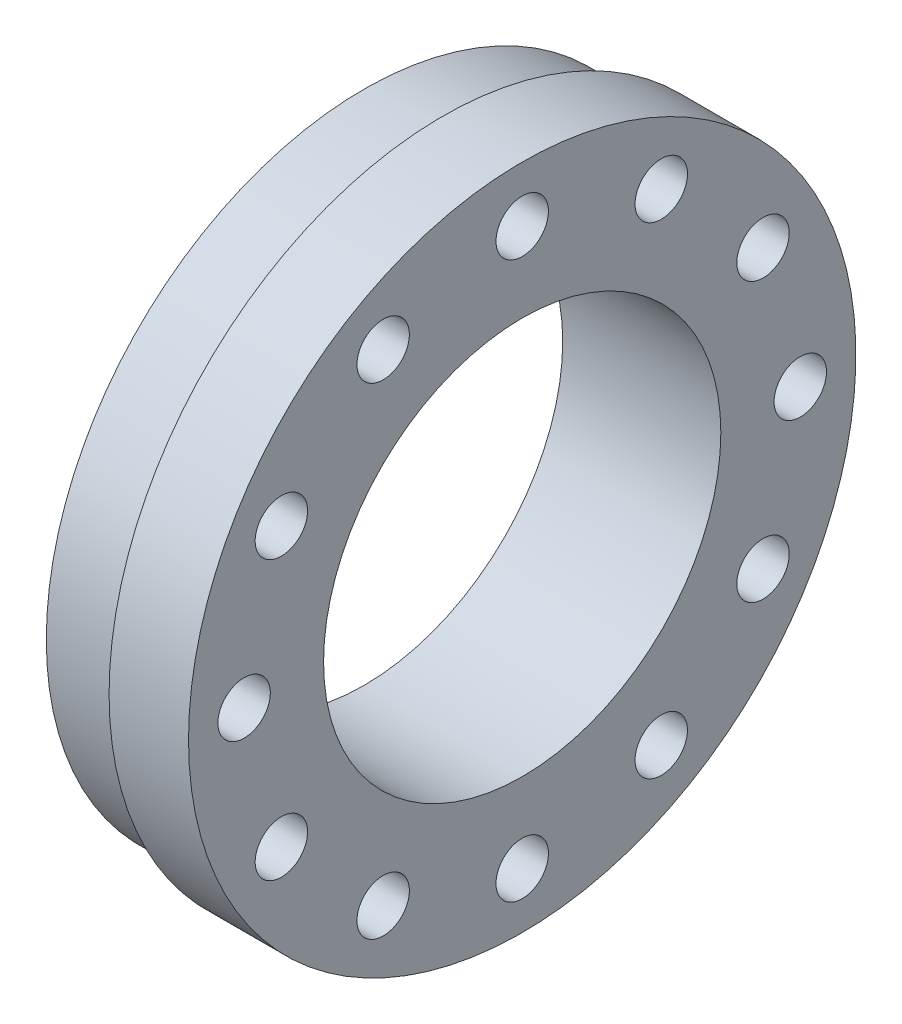
from build123d import *

# Parameters (mm, degrees)
HOLE_WIZARD_M4_1_D = 3.3


with BuildPart() as part:
    # 草图1 → 旋转1 (revolve)
    with BuildSketch(Plane(origin=(0, 0, 0), x_dir=(1, 0, 0), z_dir=(0, 1, 0)), mode=Mode.PRIVATE) as revolve_1_sk:
        Polygon((0, 12.5), (0, 20), (4.95, 20), (4.95, 21), (9.95, 21), (9.95, 12.5), align=None)
    revolve(revolve_1_sk.sketch.rotate(Axis((-63.943599205, 0, 0), (1, 0, 0)), 180), axis=Axis((-63.943599205, 0, 0), (1, 0, 0)))

    # M4 螺纹孔1 (through all)
    with Locations(Plane(origin=(9.95, 0, 0), x_dir=(0, 0, -1), z_dir=(1, 0, 0))):
        with Locations((0, 0), (0, 17.5), (8.75, 15.155444566), (15.155444566, 8.75), (17.5, 0), (15.155444566, -8.75), (8.75, -15.155444566), (0, -17.5), (-8.75, -15.155444566), (-15.155444566, -8.75), (-17.5, 0), (-15.155444566, 8.75), (-8.75, 15.155444566)):
            Hole(HOLE_WIZARD_M4_1_D / 2)


solid = part.part
